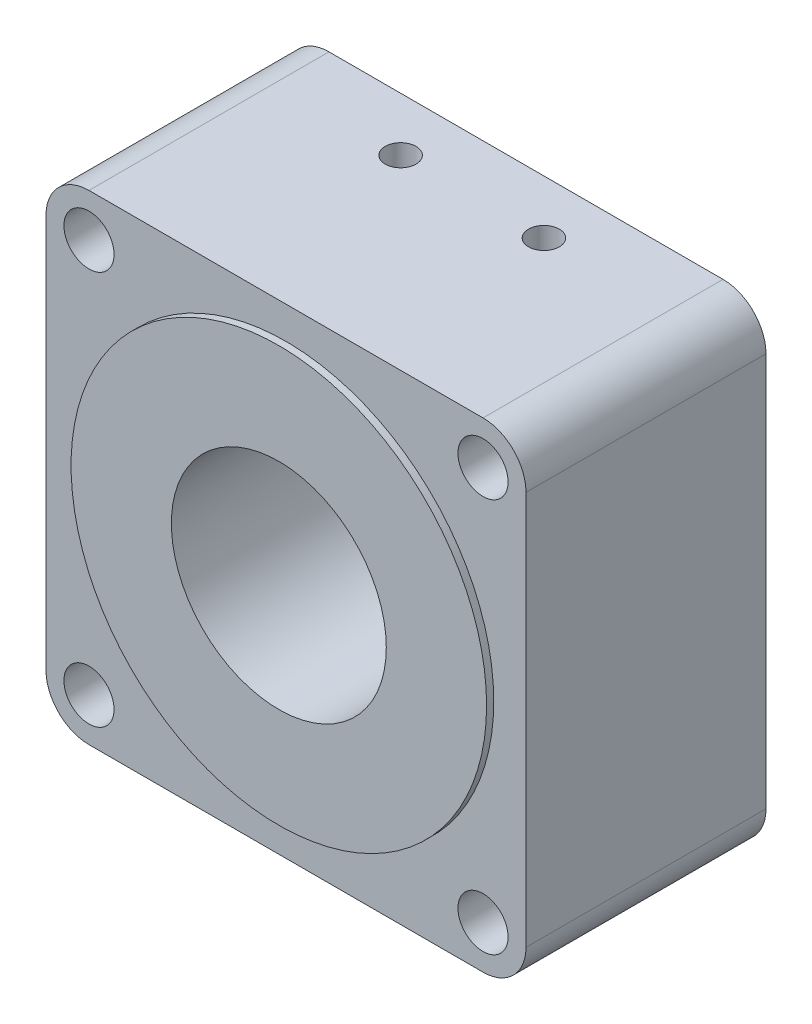
from build123d import *

# Parameters (mm, degrees)
SKETCH1_W                  = 134
SKETCH1_H                  = 134
BOSS_EXTRUDE1_DEPTH        = 67
FILLET1_R                  = 12
SKETCH2_R                  = 30
CUT_EXTRUDE1_DEPTH         = 67
BOSS_EXTRUDE2_START        = 2
SKETCH3_R                  = 58
SKETCH3_R_2                = 30
BOSS_EXTRUDE2_DEPTH        = 2
SKETCH4_R                  = 58
SKETCH4_R_2                = 30
BOSS_EXTRUDE3_DEPTH        = 2
SKETCH5_R                  = 7
CUT_EXTRUDE2_DEPTH         = 160
SKETCH6_R                  = 9.5
CUT_EXTRUDE3_DEPTH         = 40
SIZE_MM_DOWEL_HOLE_1_D     = 8.5
SIZE_MM_DOWEL_HOLE_1_DEPTH = 24.5
SIZE_MM_DOWEL_HOLE_1_TIP   = 2.553657631
SIZE_MM_DOWEL_HOLE_2_D     = 8.5
SIZE_MM_DOWEL_HOLE_2_DEPTH = 24.5
SIZE_MM_DOWEL_HOLE_2_TIP   = 2.553657631
SIZE_MM_DOWEL_HOLE_3_D     = 8.6
SIZE_MM_DOWEL_HOLE_3_DEPTH = 10
SIZE_MM_DOWEL_HOLE_3_TIP   = 2.583700662


with BuildPart() as part:
    # Sketch1 → Boss-Extrude1 (new body)
    with BuildSketch(Plane.XY):
        Rectangle(SKETCH1_W, SKETCH1_H)
    extrude(amount=BOSS_EXTRUDE1_DEPTH)

    # Fillet1
    fillet1_edges = [part.edges().sort_by_distance(p)[0] for p in [
        (-67, 67, 33.5),
        (67, 67, 33.5),
        (67, -67, 33.5),
        (-67, -67, 33.5),
    ]]
    fillet(fillet1_edges, radius=FILLET1_R)

    # Sketch2 → Cut-Extrude1 (cut)
    with BuildSketch(Plane.XY.offset(67)):
        Circle(SKETCH2_R)
    extrude(amount=-CUT_EXTRUDE1_DEPTH, mode=Mode.SUBTRACT)

    # Sketch3 → Boss-Extrude2 (add)
    with BuildSketch(Plane.XY.offset(67).offset(BOSS_EXTRUDE2_START)):
        Circle(SKETCH3_R)
        Circle(SKETCH3_R_2, mode=Mode.SUBTRACT)
    extrude(amount=-BOSS_EXTRUDE2_DEPTH)

    # Sketch4 → Boss-Extrude3 (add)
    with BuildSketch(Plane(origin=(0, 0, 0), x_dir=(-1, 0, 0), z_dir=(0, 0, -1))):
        with Locations(Location((0, 0, 0), (0, 0, 180))):
            Circle(SKETCH4_R)
        with Locations(Location((0, 0, 0), (0, 0, 180))):
            Circle(SKETCH4_R_2, mode=Mode.SUBTRACT)
    extrude(amount=BOSS_EXTRUDE3_DEPTH)

    # Sketch5 → Cut-Extrude2 (cut)
    with BuildSketch(Plane(origin=(0, 0, 0), x_dir=(-1, 0, 0), z_dir=(0, 0, -1))):
        with Locations((-55, 55)):
            Circle(SKETCH5_R)
        with Locations((55, 55)):
            Circle(SKETCH5_R)
        with Locations((55, -55)):
            Circle(SKETCH5_R)
        with Locations((-55, -55)):
            Circle(SKETCH5_R)
    extrude(amount=-CUT_EXTRUDE2_DEPTH, mode=Mode.SUBTRACT)

    # Sketch6 → Cut-Extrude3 (cut)
    with BuildSketch(Plane(origin=(0, 0, 0), x_dir=(-1, 0, 0), z_dir=(0, 0, -1))):
        with Locations((-55, 55)):
            Circle(SKETCH6_R)
        with Locations((55, 55)):
            Circle(SKETCH6_R)
        with Locations((55, -55)):
            Circle(SKETCH6_R)
        with Locations((-55, -55)):
            Circle(SKETCH6_R)
    extrude(amount=-CUT_EXTRUDE3_DEPTH, mode=Mode.SUBTRACT)

    # Size mm Dowel hole 1
    with Locations(Plane(origin=(0, 0, 0), x_dir=(-1, 0, 0), z_dir=(0, 0, -1))):
        with Locations((-36.71, 52.425), (36.71, 52.425), (36.71, -52.425), (-36.71, -52.425)):
            Hole(SIZE_MM_DOWEL_HOLE_1_D / 2, depth=SIZE_MM_DOWEL_HOLE_1_DEPTH)
            with Locations((0, 0, -(SIZE_MM_DOWEL_HOLE_1_DEPTH + SIZE_MM_DOWEL_HOLE_1_TIP / 2))):  # 118° drill point
                Cone(0, SIZE_MM_DOWEL_HOLE_1_D / 2, SIZE_MM_DOWEL_HOLE_1_TIP, mode=Mode.SUBTRACT)

    # Size mm Dowel hole 2
    with Locations(Plane(origin=(0, 0, 0), x_dir=(-1, 0, 0), z_dir=(0, 0, -1))):
        with Locations((-52.425, 36.71), (52.425, 36.71), (52.425, -36.71), (-52.425, -36.71)):
            Hole(SIZE_MM_DOWEL_HOLE_2_D / 2, depth=SIZE_MM_DOWEL_HOLE_2_DEPTH)
            with Locations((0, 0, -(SIZE_MM_DOWEL_HOLE_2_DEPTH + SIZE_MM_DOWEL_HOLE_2_TIP / 2))):  # 118° drill point
                Cone(0, SIZE_MM_DOWEL_HOLE_2_D / 2, SIZE_MM_DOWEL_HOLE_2_TIP, mode=Mode.SUBTRACT)

    # Size mm Dowel hole 3
    with Locations(Plane(origin=(0, 67, 0), x_dir=(1, 0, 0), z_dir=(0, 1, 0))):
        with Locations((-20, -15), (20, -15)):
            Hole(SIZE_MM_DOWEL_HOLE_3_D / 2, depth=SIZE_MM_DOWEL_HOLE_3_DEPTH)
            with Locations((0, 0, -(SIZE_MM_DOWEL_HOLE_3_DEPTH + SIZE_MM_DOWEL_HOLE_3_TIP / 2))):  # 118° drill point
                Cone(0, SIZE_MM_DOWEL_HOLE_3_D / 2, SIZE_MM_DOWEL_HOLE_3_TIP, mode=Mode.SUBTRACT)


solid = part.part
